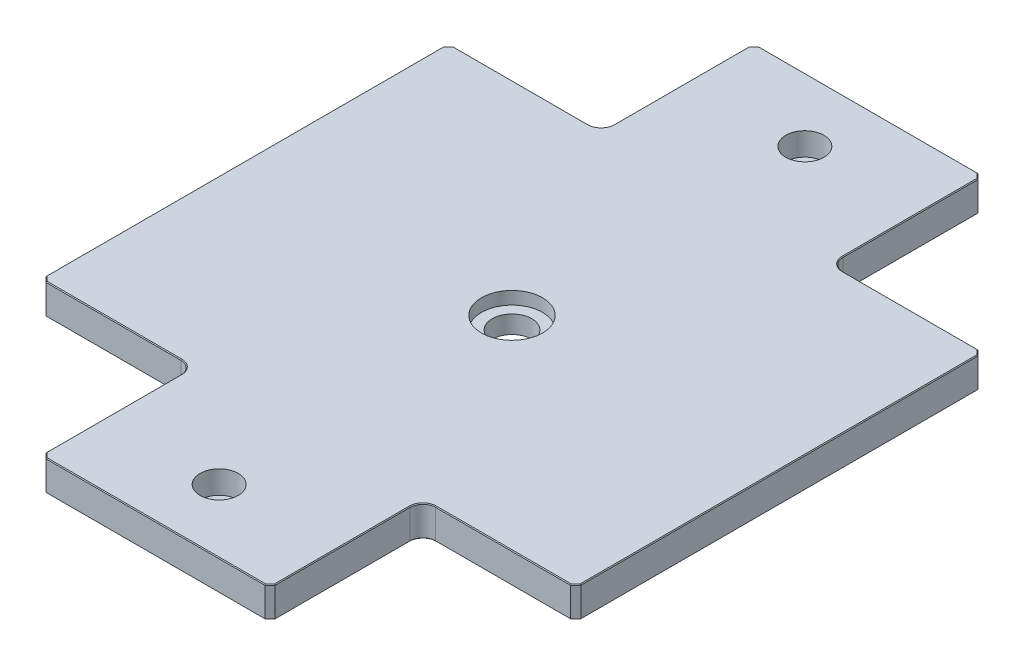
from build123d import *

# Parameters (mm, degrees)
SKETCH_1_W          = 210
SKETCH_1_H          = 280
EXTRUDE_1_DEPTH     = 12
SKETCH_2_R          = 7.75
SKETCH_2_R_2        = 4.5
CUT_EXTRUDE_1_DEPTH = 176.410946067
SKETCH_3_W          = 60
SKETCH_3_H          = 60
CUT_EXTRUDE_2_DEPTH = 176.410946067
FILLET_1_R          = 5
CHAMFER_1_SIZE      = 2
SKETCH_4_R          = 7.5
CUT_EXTRUDE_3_DEPTH = 9
SKETCH_5_R          = 12
CUT_EXTRUDE_4_DEPTH = 5
CHAMFER_2_SIZE      = 0.3
CHAMFER_3_SIZE      = 0.3


with BuildPart() as part:
    # 草图1 → 凸台-拉伸1 (new body)
    with BuildSketch(Plane(origin=(0, 0, 0), x_dir=(1, 0, 0), z_dir=(0, 1, 0))):
        Rectangle(SKETCH_1_W, SKETCH_1_H)
    extrude(amount=EXTRUDE_1_DEPTH)

    # 草图2 → 切除-拉伸1 (cut, through all)
    with BuildSketch(Plane(origin=(0, 12, 0), x_dir=(1, 0, 0), z_dir=(0, 1, 0))):
        with Locations(Location((0, 0, 0), (0, 0, 270))):
            Circle(SKETCH_2_R)
        with Locations(Location((0, -115, 0), (0, 0, 270))):
            Circle(SKETCH_2_R_2)
        with Locations(Location((0, 115, 0), (0, 0, 270))):
            Circle(SKETCH_2_R_2)
    extrude(amount=-CUT_EXTRUDE_1_DEPTH, mode=Mode.SUBTRACT)

    # 草图3 → 切除-拉伸2 (cut, through all)
    with BuildSketch(Plane(origin=(0, 12, 0), x_dir=(1, 0, 0), z_dir=(0, 1, 0))):
        with Locations((-75, -110)):
            Rectangle(SKETCH_3_W, SKETCH_3_H)
        with Locations((-75, 110)):
            Rectangle(SKETCH_3_W, SKETCH_3_H)
        with Locations((75, 110)):
            Rectangle(SKETCH_3_W, SKETCH_3_H)
        with Locations((75, -110)):
            Rectangle(SKETCH_3_W, SKETCH_3_H)
    extrude(amount=-CUT_EXTRUDE_2_DEPTH, mode=Mode.SUBTRACT)

    # 圆角1
    fillet_1_edges = [part.edges().sort_by_distance(p)[0] for p in [
        (-45, 6, 80),
        (-45, 6, -80),
        (45, 6, -80),
        (45, 6, 80),
    ]]
    fillet(fillet_1_edges, radius=FILLET_1_R)

    # 倒角1
    chamfer_1_edges = [part.edges().sort_by_distance(p)[0] for p in [
        (-105, 6, 80),
        (-45, 6, 140),
        (-105, 6, -80),
        (-45, 6, -140),
        (105, 6, -80),
        (45, 6, -140),
        (105, 6, 80),
        (45, 6, 140),
    ]]
    chamfer(chamfer_1_edges, length=CHAMFER_1_SIZE)

    # 草图4 → 切除-拉伸3 (cut)
    with BuildSketch(Plane(origin=(0, 12, 0), x_dir=(1, 0, 0), z_dir=(0, 1, 0))):
        with Locations(Location((0, -115, 0), (0, 0, 270))):
            Circle(SKETCH_4_R)
        with Locations(Location((0, 115, 0), (0, 0, 270))):
            Circle(SKETCH_4_R)
    extrude(amount=-CUT_EXTRUDE_3_DEPTH, mode=Mode.SUBTRACT)

    # 草图5 → 切除-拉伸4 (cut)
    with BuildSketch(Plane(origin=(0, 12, 0), x_dir=(1, 0, 0), z_dir=(0, 1, 0))):
        with Locations(Location((0, 0, 0), (0, 0, 270))):
            Circle(SKETCH_5_R)
    extrude(amount=-CUT_EXTRUDE_4_DEPTH, mode=Mode.SUBTRACT)

    # 倒角2
    chamfer_2_edges = [part.edges().sort_by_distance(p)[0] for p in [
        (76.5, 12, 80),
        (0, 12, 140),
        (105, 12, 0),
        (45, 12, -111.5),
        (0, 12, -140),
        (-76.5, 12, -80),
        (-105, 12, 0),
        (-45, 12, 111.5),
        (44, 12, -139),
        (104, 12, -79),
        (-44, 12, -139),
        (-104, 12, -79),
        (-104, 12, 79),
        (-44, 12, 139),
        (44, 12, 139),
        (104, 12, 79),
        (-45, 12, -111.5),
        (76.5, 12, -80),
        (45, 12, 111.5),
        (-76.5, 12, 80),
        (-46.464466094, 12, -81.464466094),
        (46.464466094, 12, -81.464466094),
        (46.464466094, 12, 81.464466094),
        (-46.464466094, 12, 81.464466094),
    ]]
    chamfer(chamfer_2_edges, length=CHAMFER_2_SIZE)

    # 倒角3
    chamfer_3_edges = [part.edges().sort_by_distance(p)[0] for p in [
        (76.5, 0, 80),
        (105, 0, 0),
        (0, 0, 140),
        (-45, 0, 111.5),
        (-105, 0, 0),
        (-76.5, 0, -80),
        (0, 0, -140),
        (45, 0, -111.5),
        (44, 0, -139),
        (104, 0, -79),
        (-44, 0, -139),
        (-104, 0, -79),
        (-104, 0, 79),
        (-44, 0, 139),
        (44, 0, 139),
        (104, 0, 79),
        (-45, 0, -111.5),
        (76.5, 0, -80),
        (45, 0, 111.5),
        (-76.5, 0, 80),
        (-46.464466094, 0, -81.464466094),
        (46.464466094, 0, -81.464466094),
        (46.464466094, 0, 81.464466094),
        (-46.464466094, 0, 81.464466094),
    ]]
    chamfer(chamfer_3_edges, length=CHAMFER_3_SIZE)


solid = part.part
